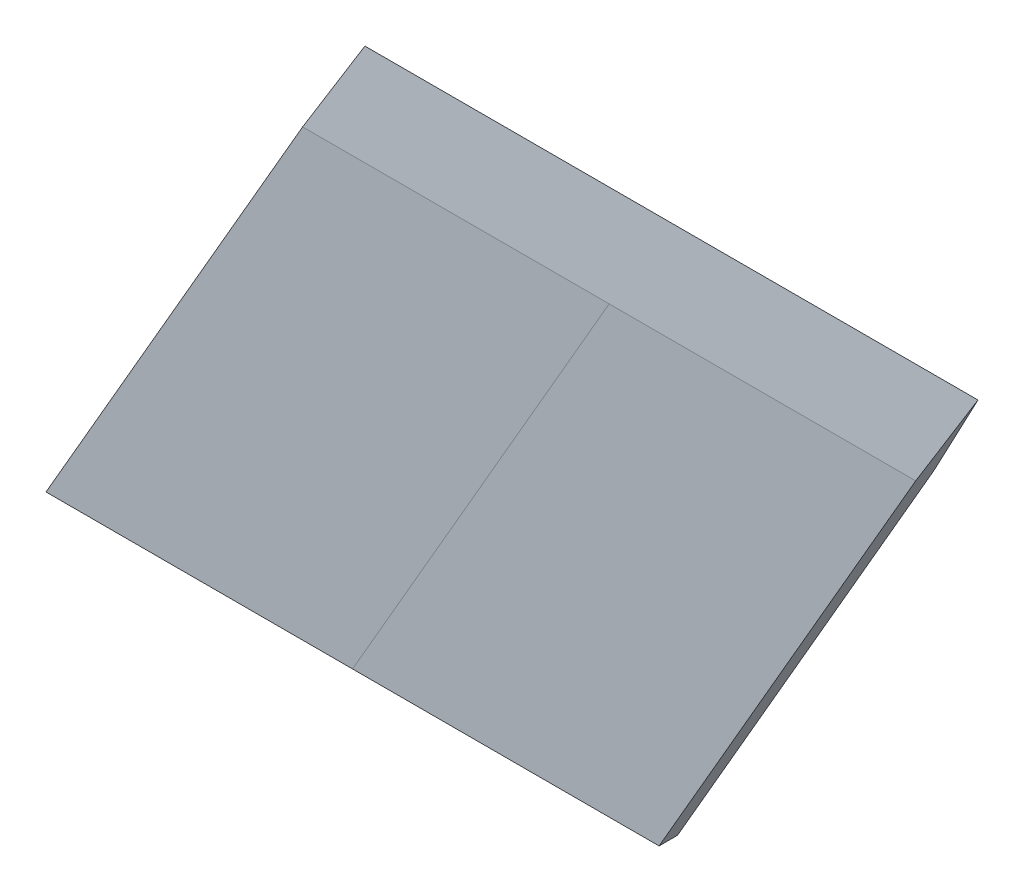
from build123d import *

# Parameters (mm, degrees)
BOSS_EXTRUDE1_DEPTH = 0.6
CUT_EXTRUDE1_DEPTH  = 35.825831243


with BuildPart() as part:
    # Sketch1 → Boss-Extrude1 (new body)
    with BuildSketch(Plane.XY):
        Polygon((0, 0), (10.103629711, 17.5), (30.103629711, 17.5), (20, 0), align=None)
    extrude(amount=BOSS_EXTRUDE1_DEPTH)

    # Sketch2 → Cut-Extrude1 (cut, through all)
    with BuildSketch(Plane(origin=(0, 0, 0), x_dir=(0, 0, -1), z_dir=(1, 0, 0))):
        Polygon((-0.3, 17.5), (0, 14.5), (0, 17.5), align=None)
    cut_extrude1 = extrude(amount=CUT_EXTRUDE1_DEPTH, mode=Mode.SUBTRACT)

    # Mirror1: Cut-Extrude1 across plane
    add(cut_extrude1.mirror(Plane(origin=(0, 0, 0.3), x_dir=(1, 0, 0), z_dir=(0, 0, -1))), mode=Mode.SUBTRACT)


solid = part.part
